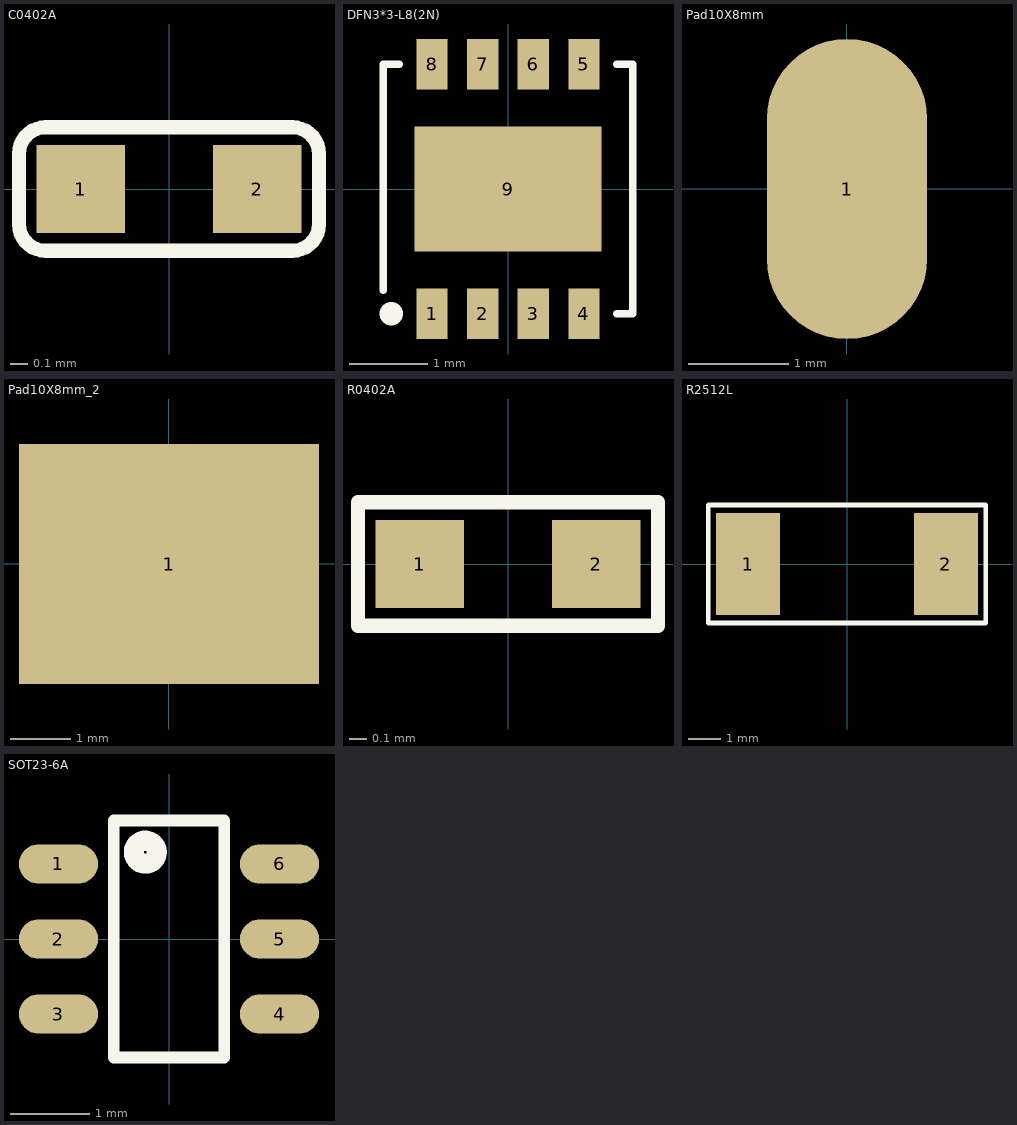
[diagram p0: the footprints below, top view; thin cyan lines are the x and y axes]
# Altium footprint library MISC78884.PcbLib: 7 footprints
Each footprint in its own frame and in the unit in brackets; x right, y up, seen from the top. Pads: shape width x height; smd on the part's side, far side on the other; paste and mask are expansions set on the pad; w line width, h text height; cw(c..) or ccw(c..) is an arc to the next point about the centre after c.

## C0402A [mm] "SMD capacitor"
pads (2):
  rect 0.5x0.5 smd paste+0 mask+0.05: 1(-0.5,0) 2(0.5,0)
Top Overlay:
  lines w0.08: -0.85,-0.2 ccw(c-0.7,-0.2) -0.7,-0.35 0.7,-0.35 ccw(c0.7,-0.2) 0.85,-0.2 0.85,0.2 ccw(c0.7,0.2) 0.7,0.35 -0.7,0.35 ccw(c-0.7,0.2) -0.85,0.2 -0.85,-0.2

## DFN3*3-L8(2N) [mm] "DFN3*3 dual SMD MOS"
height 2.5
pads (9):
  rect 0.4x0.65 smd: 1(-0.975,-1.6) 2(-0.325,-1.6) 3(0.325,-1.6) 4(0.975,-1.6) 5(0.975,1.6) 6(0.325,1.6) 7(-0.325,1.6) 8(-0.975,1.6)
  rect 2.4x1.6 smd: 9(0,0)
Top Overlay:
  lines w0.1: -1.6,-1.3 -1.6,1.6 -1.4,1.6 ; 1.4,-1.6 1.6,-1.6 1.6,1.6 1.4,1.6
  lines w0.3: -1.5,-1.6 -1.5,-1.597

## Pad10X8mm [mm]
pads (1):
  oval 1.6x3 smd: 1(0,0)

## Pad10X8mm_2 [mm]
pads (1):
  rect 5x4 smd: 1(0,0)

## R0402A [mm] "SMD resistor"
pads (2):
  rect 0.5x0.5 smd paste+0 mask+0.05: 1(-0.5,0) 2(0.5,0)
Top Overlay:
  lines w0.08: -0.85,-0.35 0.85,-0.35 0.85,0.35 -0.85,0.35 -0.85,-0.35

## R2512L [mm] "SMD resistor"
pads (2):
  rect 2x3.2 smd: 1(-3.1,0) 2(3.1,0)
Top Overlay:
  lines w0.15: -4.35,-1.85 -4.35,1.85 4.35,1.85 4.35,-1.85 -4.35,-1.85

## SOT23-6A [mm]
pads (6):
  oval 1x0.5 smd mask+0.05: 1(-1.4,0.95) 2(-1.4,0) 3(-1.4,-0.95) 4(1.4,-0.95) 5(1.4,0) 6(1.4,0.95)
Top Overlay:
  circle w0.254: c-0.3,1.1 r0.146
  lines w0.15: -0.7,-1.5 0.7,-1.5 0.7,1.5 -0.7,1.5 -0.7,-1.5